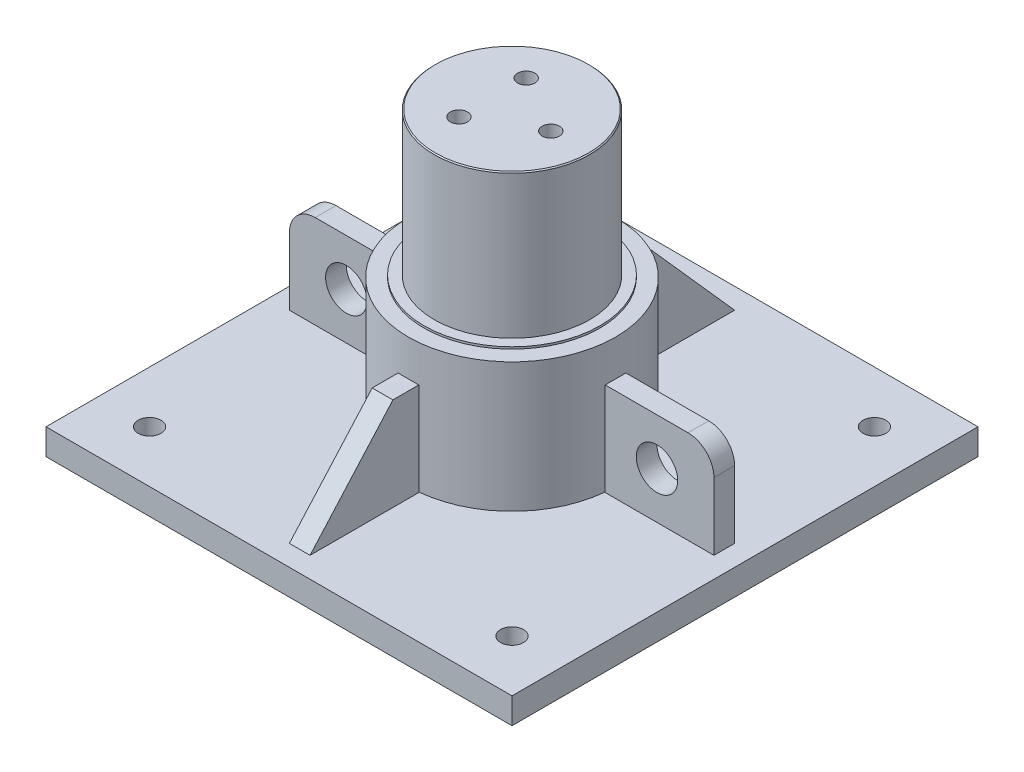
SolidWorks part; units mm, degrees
material "Plain Carbon Steel"
ref_plane "Front Plane" through (0, 0, 0) normal (0, 0, 1) x (1, 0, 0)
ref_plane "Top Plane" through (0, 0, 0) normal (0, 1, 0) x (1, 0, 0)
ref_plane "Right Plane" through (0, 0, 0) normal (1, 0, 0) x (0, 0, -1)
sketch "Sketch1" plane through (0, 0, 0) normal (0, 1, 0) x (1, 0, 0)
  line L1 (-225, 225) -> (225, 225)
  line L2 (-225, 225) -> (-225, -225)
  line L3 (-225, -225) -> (225, -225)
  line L4 (225, 225) -> (225, -225)
  line L5 (-225, 225) -> (225, -225) construction
  line L6 (-225, -225) -> (225, 225) construction
  circle A0 centre (0, 0) radius 100
  point P0 (0, 0)
  dimension "D2" = 200
  dimension "D1" = 450
extrude "Boss-Extrude1" add sketch "Sketch1" along normal blind 25
sketch "Sketch2" plane through (0, 0, 0) normal (0, -1, 0) x (1, 0, 0)
  circle A0 centre (0, 0) radius 100 construction
  circle A1 centre (0, 0) radius 100
extrude "Boss-Extrude2" add sketch "Sketch2" against normal blind 150 separate body
sketch "Sketch3" plane through (0, 150, 0) normal (0, 1, 0) x (1, 0, 0)
  circle A0 centre (0, 0) radius 85
  dimension "D1" = 170
extrude "Boss-Extrude3" add sketch "Sketch3" along normal blind 2
sketch "Sketch4" plane through (0, 152, 0) normal (0, 1, 0) x (1, 0, 0)
  circle A0 centre (0, 0) radius 75
  dimension "D1" = 150
extrude "Boss-Extrude4" add sketch "Sketch4" along normal blind 139
sketch "Sketch5" plane through (0, 25, 0) normal (0, 1, 0) x (1, 0, 0)
  line L0 (-225, 0) -> (225, 0) construction
  line L1 (-225, 225) -> (-225, -225) construction
  line L2 (225, -225) -> (225, 225) construction
  line L3 (0, 225) -> (0, -225) construction
  line L4 (225, 225) -> (-225, 225) construction
  line L5 (-225, -225) -> (225, -225) construction
  line L6 (-175, 225) -> (-175, -225) construction
  line L7 (-225, -175) -> (225, -175) construction
  line L8 (175, 225) -> (175, -225) construction
  line L9 (-225, 175) -> (225, 175) construction
  circle A0 centre (-175, 175) radius 11
  circle A1 centre (175, 175) radius 11
  circle A2 centre (175, -175) radius 11
  circle A3 centre (-175, -175) radius 11
  dimension "D3" = 22
  dimension "D1" = 175
  dimension "D2" = 175
extrude "Cut-Extrude1" cut sketch "Sketch5" against normal through all
sketch "Sketch6" plane through (0, 291, 0) normal (0, 1, 0) x (1, 0, 0)
  line L0 (0, 0) -> (37.5, 0) construction
  circle A0 centre (0, 0) radius 37.5 construction
  dimension "D1" = 75
hole_wizard "3/4-10 Tapped Hole1" positions "3DSketch1" profile "Sketch7" tap size "3/4-10" standard "ANSI Inch"
sketch3d "3DSketch1"
  point P0 (37.5, 291, 0)
sketch "Sketch7" plane through (37.5, 291, 0) normal (1, 0, 0) x (0, 0, 1)
  line L0 (0, 0) -> (0, 35.0074)
  line L1 (0, 35.0074) -> (8.3337, 30)
  line L2 (8.3337, 30) -> (8.3337, 0)
  line L5 (8.3337, 0) -> (0, 0)
  line L10 (0, 35.0074) -> (-8.3337, 30) construction
  line L11 (0, -6.35) -> (0, 107.95) construction
  dimension "Tap Drill Dia." = 16.6675
  dimension "Tap Drill Depth" = 30
  dimension "Drill Angle" = 118
cosmetic thread "Hole Thread1" parameters "D1"=30, "D2"=19.05
pattern_circular "CirPattern1" count 3 over 360 about axis through (0, 0, 0) along (0, 1, 0) of "3/4-10 Tapped Hole1"
chamfer "Chamfer1" distance 1 angle 45 1 edges at (0, 291, 75)
sketch "Sketch8" plane through (0, 0, 0) normal (0, 0, 1) x (1, 0, 0)
  line L0 (-205, 25) -> (-205, 115)
  line L1 (-225, 25) -> (225, 25) construction
  line L2 (-205, 115) -> (-100, 115)
  line L3 (-100, 115) -> (-100, 25)
  line L4 (-100, 25) -> (-205, 25)
  line L5 (-225, 25) -> (-225, 0) construction
  line L6 (0, 0) -> (0, 315.8837) construction
  line L7 (-225, 0) -> (225, 0) construction
  line L8 (100, 25) -> (205, 25)
  line L9 (100, 115) -> (100, 25)
  line L10 (205, 115) -> (100, 115)
  line L11 (205, 25) -> (205, 115)
  point P5 (-225, 12.5)
  dimension "D1" = 105
  dimension "D2" = 90
  dimension "D3" = 20
extrude "Boss-Extrude5" add sketch "Sketch8" along normal mid plane 20 separate body
fillet "Fillet1" radius 25 1 edges at (-205, 115, 0)
fillet "Fillet2" radius 25 1 edges at (205, 115, 0)
sketch "Sketch9" plane through (0, 0, 10) normal (0, 0, 1) x (1, 0, 0)
  line L0 (-150, 11.9434) -> (-150, 128.0566) construction
  line L1 (-81.1129, 70) -> (-230.7523, 70) construction
  line L2 (-225, 0) -> (225, 0) construction
  line L3 (-100, 150) -> (-100, 0) construction
  line L4 (0, 0) -> (0, 320.562) construction
  line L5 (81.1129, 70) -> (230.7523, 70) construction
  line L6 (150, 11.9434) -> (150, 128.0566) construction
  circle A0 centre (-150, 70) radius 20
  circle A1 centre (150, 70) radius 20
  dimension "D3" = 40
  dimension "D1" = 70
  dimension "D2" = 50
extrude "Cut-Extrude2" cut sketch "Sketch9" against normal through all both and the other way through all
sketch "Sketch10" plane through (0, 0, 0) normal (1, 0, 0) x (0, 0, -1)
  line L0 (-100, 25) -> (-205, 25)
  line L1 (-225, 25) -> (225, 25) construction
  line L2 (-100, 150) -> (-100, 0) construction
  line L3 (-205, 25) -> (-125, 115)
  line L4 (-125, 115) -> (-100, 115)
  line L5 (-100, 115) -> (-100, 25)
  line L6 (0, 0) -> (0, 203.5377) construction
  line L7 (-225, 0) -> (225, 0) construction
  line L8 (100, 115) -> (100, 25)
  line L9 (125, 115) -> (100, 115)
  line L10 (205, 25) -> (125, 115)
  line L11 (100, 25) -> (205, 25)
  dimension "D1" = 25
  dimension "D2" = 20
  dimension "D3" = 90
extrude "Boss-Extrude6" add sketch "Sketch10" along normal mid plane 20 separate body
